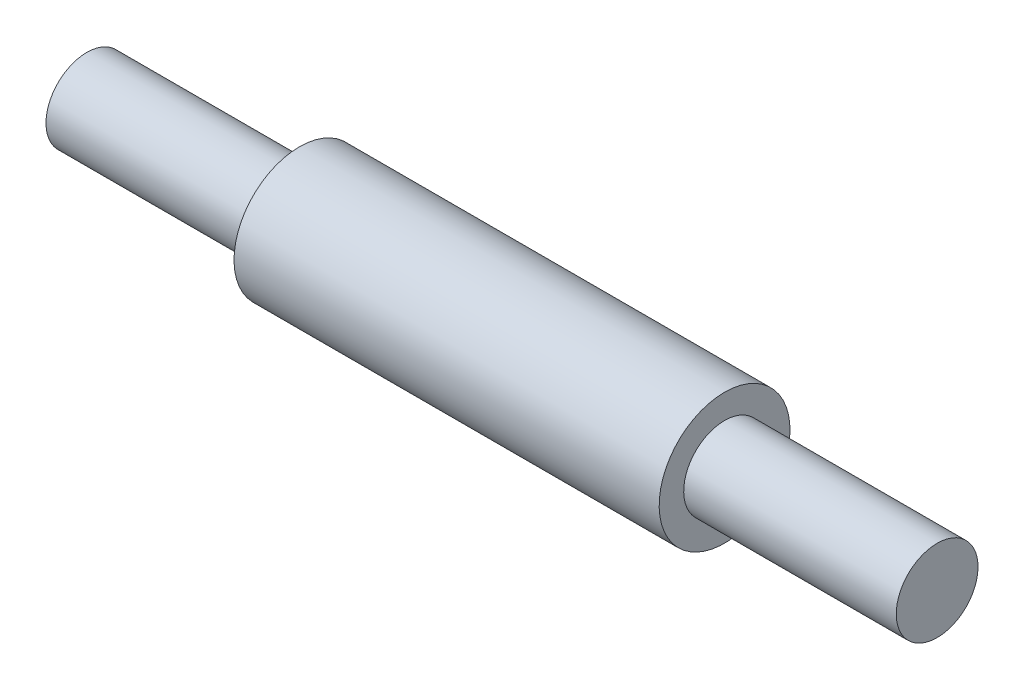
SolidWorks part; units mm, degrees
ref_plane "Front Plane" through (0, 0, 0) normal (0, 0, 1) x (1, 0, 0)
ref_plane "Top Plane" through (0, 0, 0) normal (0, 1, 0) x (1, 0, 0)
ref_plane "Right Plane" through (0, 0, 0) normal (1, 0, 0) x (0, 0, -1)
sketch "Sketch1" plane through (0, 0, 0) normal (0, 0, 1) x (1, 0, 0)
  line L0 (26, 0) -> (-26, 0)
  line L1 (-26, 0) -> (-26, 2.5)
  line L2 (-26, 2.5) -> (-13, 2.5)
  line L3 (-13, 2.5) -> (-13, 4)
  line L4 (-13, 4) -> (13, 4)
  line L5 (13, 4) -> (13, 2.5)
  line L6 (13, 2.5) -> (26, 2.5)
  line L7 (26, 2.5) -> (26, 0)
  dimension "D1" = 52
  dimension "D2" = 2.5
  dimension "D3" = 26
  dimension "D4" = 4
revolve "Revolve1" add sketch "Sketch1" angle 360 about L0
